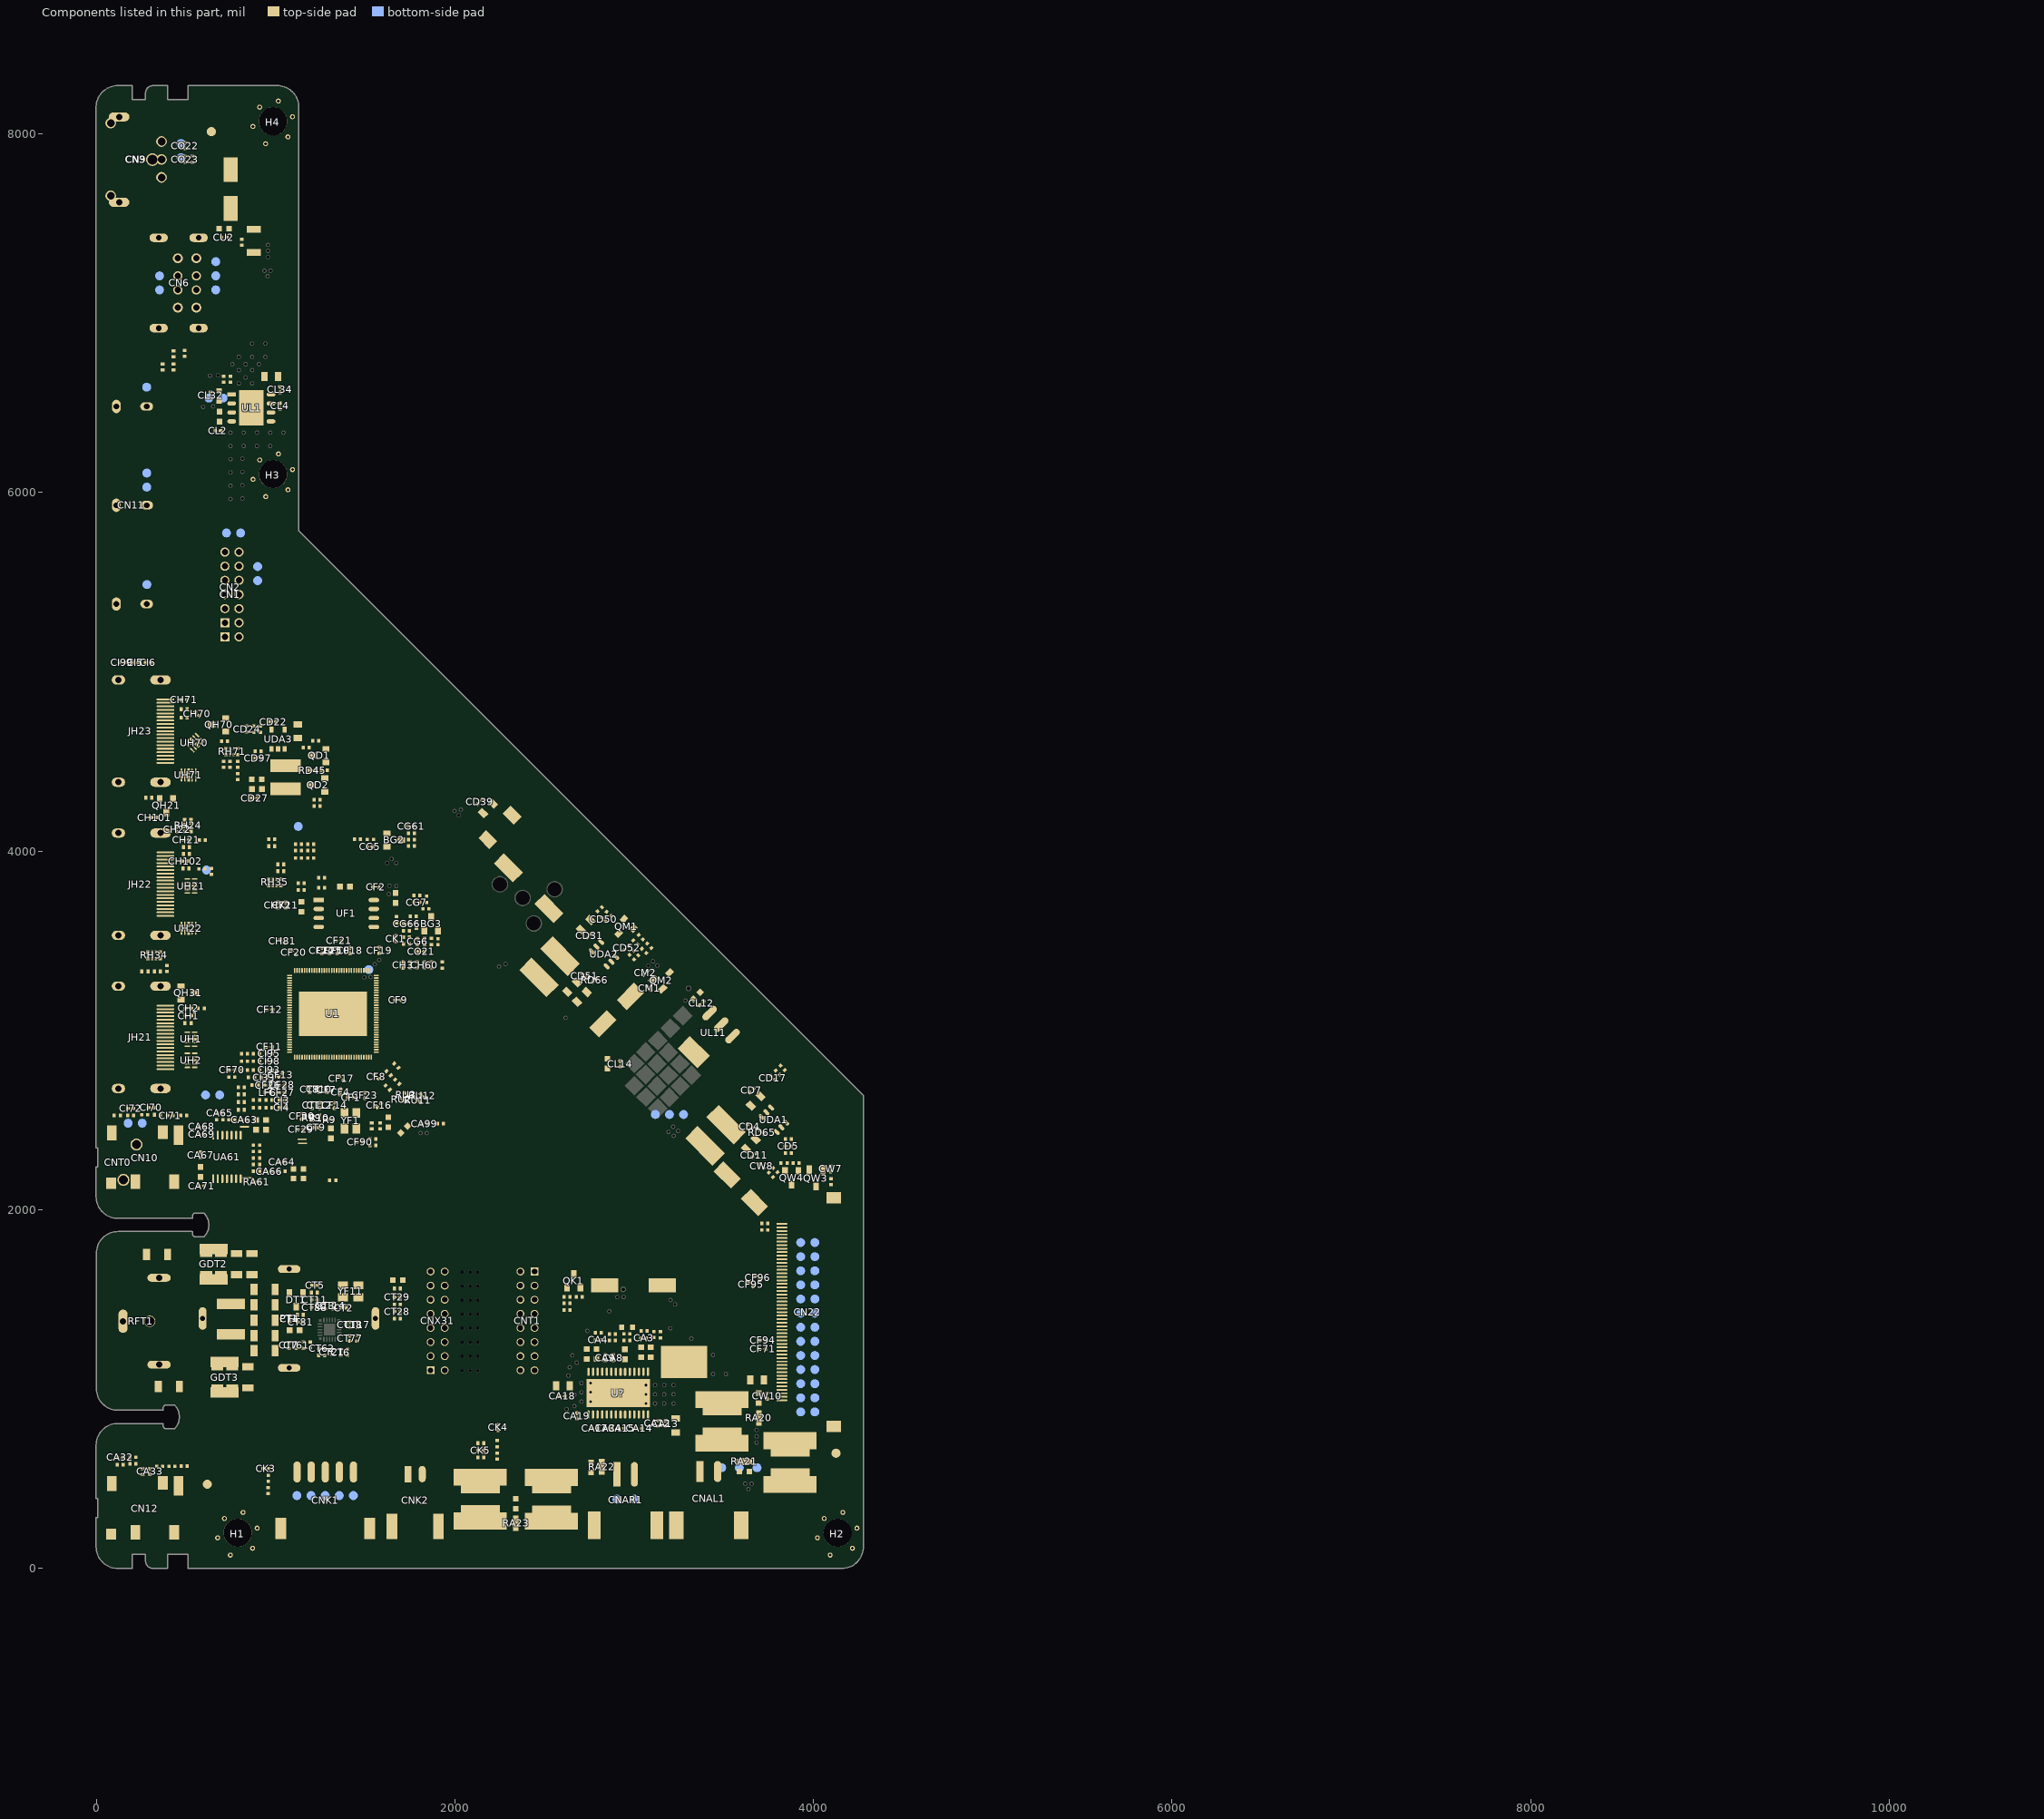
[diagram p0: the components of this part, seen from the top]
# Altium PCB MISC105950.PcbDoc (part 4 of 15)
Units mil, origin at the board's own origin, x right, y up, seen from the top; angles counter-clockwise.
Board outline 4280.62 x 8272.76 mil, 2 copper layers (TopLayer, BottomLayer), stack 61.855 mil thick; 541 components, 268 nets, 2324 pads, 1157 vias.

## Footprints (in the part's own frame and the unit in brackets; to place one, negate y for a bottom-side part, rotate by r counter-clockwise, add the part's x,y. Pads: shape width x height; smd on the part's side, far side on the other; paste and mask are expansions set on the pad) (continued)
QFN128/0.35-1 [mm] "Mstar,TSUMV53RWUT-Z1,18.11.16(19.03.30   减少外延焊盘长度）(19.04.23 更新钢网尺寸）（因温升修改为12宫格）"
  oct 2.2x1.9 on Top Paste: 0(-3.7,0) 0(-3.697,-2.145) 0(-3.697,2.145) 0(-1.253,-2.145) 0(-1.253,2.145) 0(-1.25,0) 0(1.247,-2.145) 0(1.247,2.145) 0(1.25,0) 0(3.697,-2.145) 0(3.697,2.145) 0(3.7,0)
  oct 2.2x1.9 on Top Solder: 0(-3.7,0) 0(-3.697,-2.145) 0(-3.697,2.145) 0(-1.253,-2.145) 0(-1.253,2.145) 0(-1.25,0) 0(1.247,-2.145) 0(1.247,2.145) 0(1.25,0) 0(3.697,-2.145) 0(3.697,2.145) 0(3.7,0)
  rect 0.7x0.22 smd paste-0.02 mask-0.035: 1(-6.151,5.425)
  oval 0.7x0.22 smd paste-0.02 mask-0.035: 2(-6.151,5.075) 3(-6.151,4.725) 4(-6.151,4.375) 5(-6.151,4.025) 6(-6.151,3.675) 7(-6.151,3.325) 8(-6.151,2.975) 9(-6.151,2.625) 10(-6.151,2.275) 11(-6.151,1.925) 12(-6.151,1.575) 13(-6.151,1.225) 14(-6.151,0.875) 15(-6.151,0.525) 16(-6.151,0.175) 17(-6.151,-0.175) 18(-6.151,-0.525) 19(-6.151,-0.875) 20(-6.151,-1.225) 21(-6.151,-1.575) 22(-6.151,-1.925) 23(-6.151,-2.275) 24(-6.151,-2.625) 25(-6.151,-2.975) 26(-6.151,-3.325) 27(-6.151,-3.675) 28(-6.151,-4.025) 29(-6.151,-4.375) 30(-6.151,-4.725) 31(-6.151,-5.075) 32(-6.151,-5.425) 65(6.151,-5.425) 66(6.151,-5.075) 67(6.151,-4.725) 68(6.151,-4.375) 69(6.151,-4.025) 70(6.151,-3.675) 71(6.151,-3.325) 72(6.151,-2.975) 73(6.151,-2.625) 74(6.151,-2.275) 75(6.151,-1.925) 76(6.151,-1.575) 77(6.151,-1.225) 78(6.151,-0.875) 79(6.151,-0.525) 80(6.151,-0.175) 81(6.151,0.175) 82(6.151,0.525) 83(6.151,0.875) 84(6.151,1.225) 85(6.151,1.575) 86(6.151,1.925) 87(6.151,2.275) 88(6.151,2.625) 89(6.151,2.975) 90(6.151,3.325) 91(6.151,3.675) 92(6.151,4.025) 93(6.151,4.375) 94(6.151,4.725) 95(6.151,5.075) 96(6.151,5.425)
  oval 0.22x0.7 smd paste-0.02 mask-0.035: 33(-5.425,-6.151) 34(-5.075,-6.151) 35(-4.725,-6.151) 36(-4.375,-6.151) 37(-4.025,-6.151) 38(-3.675,-6.151) 39(-3.325,-6.151) 40(-2.975,-6.151) 41(-2.625,-6.151) 42(-2.275,-6.151) 43(-1.925,-6.151) 44(-1.575,-6.151) 45(-1.225,-6.151) 46(-0.875,-6.151) 47(-0.525,-6.151) 48(-0.175,-6.151) 49(0.175,-6.151) 50(0.525,-6.151) 51(0.875,-6.151) 52(1.225,-6.151) 53(1.575,-6.151) 54(1.925,-6.151) 55(2.275,-6.151) 56(2.625,-6.151) 57(2.975,-6.151) 58(3.325,-6.151) 59(3.675,-6.151) 60(4.025,-6.151) 61(4.375,-6.151) 62(4.725,-6.151) 63(5.075,-6.151) 64(5.425,-6.151) 97(5.425,6.151) 98(5.075,6.151) 99(4.725,6.151) 100(4.375,6.151) 101(4.025,6.151) 102(3.675,6.151) 103(3.325,6.151) 104(2.975,6.151) 105(2.625,6.151) 106(2.275,6.151) 107(1.925,6.151) 108(1.575,6.151) 109(1.225,6.151) 110(0.875,6.151) 111(0.525,6.151) 112(0.175,6.151) 113(-0.175,6.151) 114(-0.525,6.151) 115(-0.875,6.151) 116(-1.225,6.151) 117(-1.575,6.151) 118(-1.925,6.151) 119(-2.275,6.151) 120(-2.625,6.151) 121(-2.975,6.151) 122(-3.325,6.151) 123(-3.675,6.151) 124(-4.025,6.151) 125(-4.375,6.151) 126(-4.725,6.151) 127(-5.075,6.151) 128(-5.425,6.151)
  rect 9.6x6.3 smd paste-6 mask-6: EPAD(0,0)
  silkscreen extent -7.48,-7.42 7.42,7.4, body extent -6.2,-6.2 6.2,6.2, height 0.95
R0402 [mm] "片式电阻"
  rect 0.45x0.5 smd mask+0.076: 1(-0.425,0) 2(0.425,0)
  silkscreen extent -0.8,-0.4 0.8,0.4, body extent -0.5,-0.25 0.5,0.25, height 0.5
R0402SC#1 [mm]
  rect 0.45x0.5 smd mask+0.076: 1(-0.425,0) 2(0.425,0)
  rect 0.42x0.25 smd paste-0.5 mask-0.5: 3(0,0)
  silkscreen extent -0.8,-0.4 0.8,0.4, body extent -0.5,-0.25 0.5,0.25, height 0.5
R0402SC#2 [mm]
  rect 0.45x0.5 smd mask+0.076: 1(-0.425,0) 2(0.425,0)
  rect 0.42x0.305 smd paste-0.5 mask-0.5: 3(0,0)
  silkscreen extent -0.8,-0.4 0.8,0.4, body extent -0.5,-0.25 0.5,0.25, height 0.5
R0603 [mm] "贴片电阻"
  rect 0.7x0.8 smd mask+0.076: 1(-0.756,0) 2(0.756,0)
  silkscreen extent -1.25,-0.54 1.25,0.54, body extent -0.8,-0.4 0.8,0.4, height 0.8
R0603SC [mm] "贴片电阻"
  rect 0.7x0.8 smd mask+0.076: 1(-0.756,0) 2(0.756,0)
  rect 0.82x1 smd paste-0.5 mask-0.5: 3(0,0)
  silkscreen extent -1.25,-0.54 1.25,0.54, body extent -0.8,-0.4 0.8,0.4, height 0.8
RA0402 [mm] "排阻"
  rect 0.5x0.5 smd mask+0.076: 1(-0.45,0.85) 2(0.45,0.85) 7(-0.45,-0.85) 8(0.45,-0.85)
  rect 0.5x0.3 smd mask+0.076: 3(-0.45,0.25) 4(0.45,0.25) 5(-0.45,-0.25) 6(0.45,-0.25)
  silkscreen extent -0.85,-1.27 0.85,1.27, body extent -0.51,-1 0.51,1, height 0.35
RCL0524P [mm] "RCLAMP0524J(19.03.04 优化丝印）"
  rect 0.21x0.8 smd: 1(-1,-0.52)
  oval 0.21x0.8 smd: 2(-0.5,-0.52) 3(0.5,-0.52) 4(1,-0.52) 5(1,0.52) 6(0.5,0.52) 7(-0.5,0.52) 8(-1,0.52)
  rect 0.38x0.8 smd: GND(0,0.52) GND(0,-0.52)
  silkscreen extent -1.4,-2.03 1.4,1.14, body extent -1.25,-0.6 1.25,0.6, height 0.66
SHIELD(24.5*14*6)-TEMP-NG [mm] "屏蔽罩"
  rect 2.8x5.5 on Top Paste mask+0.051: 0(-7,0) 0(7,0)
  rect 5.5x2.8 on Top Paste mask+0.051: 0(0,12.25) 0(0,-12.25)
  oval 3.2x1.1 hole 0.7 slot 2.8 at 0 deg mask+0.051: 1(0,12.25) 2(0,-12.25)
  oval 1.1x3.2 hole 0.7 slot 2.8 at 90 deg mask+0.051: 3(7,0) 4(-7,0)
  silkscreen extent -7.48,-13.1 7.51,13.1, body extent -7.53,-13.17 7.53,13.16, height 6.1
SIP2*6H/2.0D-LS [mm] "新富尔，PHD-2*6AW-DK-SMT-P，带扣、台阶。XXXXXXXXXXXXXX项目用，17.08.16"
  rect 1.75x2.45 on Top Paste: 0(-5,-1.365) 0(-5,1.388) 0(-3,-1.364) 0(-3,1.388) 0(-1,-1.364) 0(-1,1.388) 0(1,-1.365) 0(1,1.388) 0(3,1.388) 0(3,-1.365) 0(5,-1.365) 0(5,1.388)
  rect 1.3x1.3 hole 0.9 mask+0.076: 1(-5,0.788)
  round 1.3 hole 0.9 mask+0.076: 2(-5,-1.212) 3(-3,0.788) 4(-3,-1.212) 5(-1,0.788) 6(-1,-1.212) 7(1,0.787) 8(1,-1.212) 9(3,0.788) 10(3,-1.212) 11(5,0.788) 12(5,-1.212)
  silkscreen extent -7.82,-9.54 7.1,2.41
SIP2*7H/2.0D-LS [mm] "新富尔，PHD-2*7AW-DK-SMT-P，带卡扣、台阶。XXXXXXXXXXXXXX项目用，17.08.16"
  rect 1.75x2.45 on Top Paste: 0(-6,-1.365) 0(-6,1.388) 0(-4,-1.364) 0(-4,1.388) 0(-2,-1.364) 0(-2,1.388) 0(0,1.388) 0(0,-1.365) 0(2,1.388) 0(2,-1.365) 0(4,-1.365) 0(4,1.388) 0(6,-1.364) 0(6,1.388)
  rect 1.3x1.3 hole 0.9 mask+0.076: 1(-6,0.788)
  round 1.3 hole 0.9 mask+0.076: 2(-6,-1.212) 3(-4,0.788) 4(-4,-1.212) 5(-2,0.788) 6(-2,-1.212) 7(0,0.787) 8(0,-1.212) 9(2,0.788) 10(2,-1.212) 11(4,0.788) 12(4,-1.212) 13(6,0.788) 14(6,-1.212)
  silkscreen extent -8.82,-9.54 8.1,2.41
SIP2*8H/2.0DF-1 [mm] "东莞龙科；130-F1628210-B91;15.02.06"
  round 1.3 on Top Overlay: 0(-7,-1) 0(-5,-1) 0(-5,1) 0(-3,-1) 0(-3,1) 0(-1,-1) 0(-1,1) 0(1,-1) 0(1,1) 0(3,-1) 0(3,1) 0(5,-1) 0(5,1) 0(7,-1) 0(7,1)
  rect 1.3x1.3 on Top Overlay: 0(-7,1)
  rect 1.1x1.1 hole 0.8: 1(-7,1)
  round 1.1 hole 0.8: 2(-7,-1) 3(-5,1) 4(-5,-1) 5(-3,1) 6(-3,-1) 7(-1,1) 8(-1,-1) 9(1,1) 10(1,-1) 11(3,1) 12(3,-1) 13(5,1) 14(5,-1) 15(7,1) 16(7,-1)
  silkscreen extent -8.75,-8.9 8.35,2.54, body extent -8.25,-8.8 8.25,1.2, height 6.03
SIP2*8H/2.0DM-1 [mm] "东莞龙科；142-M1628210-B31;15.02.06"
  round 1.3 on Top Overlay: 0(-7,-1) 0(-5,-1) 0(-5,1) 0(-3,1) 0(-3,-1) 0(-1,1) 0(-1,-1) 0(1,1) 0(1,-1) 0(3,1) 0(3,-1) 0(5,-1) 0(5,1) 0(7,-1) 0(7,1)
  rect 1.3x1.3 on Top Overlay: 0(-7,1)
  rect 1.1x1.1 hole 0.8: 1(-7,1)
  round 1.1 hole 0.8: 2(-7,-1) 3(-5,1) 4(-5,-1) 5(-3,1) 6(-3,-1) 7(-1,1) 8(-1,-1) 9(1,1) 10(1,-1) 11(3,1) 12(3,-1) 13(5,1) 14(5,-1) 15(7,1) 16(7,-1)
  silkscreen extent -11.73,-7.87 11.73,2.54, body extent -11.6,-7.77 11.6,1.23, height 5.5
SIP2H/2.0S-3 [mm] "捷仕泰/铭锋达/创佳；2PIN-2.0-L-M-G-带扣-带台阶-C；14.07.28"
  rect 1x2.3 smd: 1(-1,3.7)
  oval 1x2.3 smd: 2(1,3.7)
  rect 1.5x3.6 smd: 3(-3.3,-3.7) 4(3.3,-3.7)
  silkscreen extent -4.13,-5.15 4.13,4.15
SIP2H/2.5S-3 [mm] "新富尔；XH-2AWB-DK-R;插线高度为9.8mm;15.08.31"
  rect 1x3.5 smd: 1(-1.25,1)
  oval 1x3.5 smd: 2(1.25,1)
  rect 1.8x3.9 smd: 3(4.45,-6.2) 4(-4.45,-6.2)
  silkscreen extent -5.13,-7.95 5.13,0.05
SIP2H/2.5S-4 [mm] "正理；TJC3B-2AW(插线后高度8.5mm)；160607"
  rect 1x3 smd: 1(-1.25,1.4)
  oval 1x3 smd: 2(1.25,1.4)
  rect 2.1x3.9 smd: 3(4.6,-6.2) 4(-4.6,-6.2)
  silkscreen extent -5.15,-7.95 5.15,0.1
SIP5H/2.0S-4 [mm] "浙江正理；2008-nAW-S;15.07.27(17.06.16缩小优化地脚焊盘）"
  oval 1x3 smd: 1(-4,4) 2(-2,4) 3(0,4) 4(2,4) 5(3.997,3.997)
  rect 1.5x3 smd: 6(6.3,-4) 7(-6.3,-4)
  silkscreen extent -7.18,-5.27 7.18,4.1, body extent -7,-5.1 7,5, height 5.18
SMD4532-1 [mm] "Brightking,4532-091-LF,气体放电管,雷电防护器件，17.06.12"
  rect 1.5x4 smd: 1(-2.15,0) 2(2.151,0)
  silkscreen extent -1.25,-1.79 1.23,1.71, body extent -2.41,-1.75 2.41,1.75, height 3
SMD4532-1-C1206 [mm] "Brightking,4532-091-LF,SMD4532-1兼容C1206封装，19.01.08"
  rect 1.6x1 smd paste-5 mask-5: 1(-1.016,-1.501) 1(1.016,-1.499) 2(-1.016,1.501) 2(1.016,1.501)
  rect 1.6x1 on Top Paste paste-5 mask-5: 1(-1.016,-1.501) 1(1.016,-1.501) 2(-1.016,1.501) 2(1.016,1.501)
  rect 4x1.5 smd paste-5 mask-5: 1(0,-2.15) 2(0,2.151)
  rect 4.001x0.903 on Top Paste: 1(0.05,-2.499) 2(0.05,2.499)
  silkscreen extent -1.96,-1.16 1.96,1.2, body extent -1.82,-2.41 1.81,2.41, height 3
SO-23 [mm] "双向二极管封装"
  rect 0.8x1 smd: 1(0.952,1.016) 3(-0.953,1.016)
  rect 0.8x1.1 smd: 2(0,-0.966)
  silkscreen extent -1.55,-0.86 1.55,0.36, body extent -1.5,-1.25 1.5,1.25, height 1.1
SOIC8 [mm] "W25X40BVSNIG/GD25Q32BSIG/GD25LQ16"
  rect 1.5x0.6 smd: 1(-3.9,1.905)
  oval 1.5x0.6 smd: 2(-3.9,0.635) 3(-3.9,-0.635) 4(-3.9,-1.905) 5(3.9,-1.905) 6(3.9,-0.635) 7(3.9,0.635) 8(3.9,1.905)
  silkscreen extent -5.71,-2.65 2.7,2.65, body extent -4.05,-2.69 4.05,2.69, height 2.17
SOP8/1.27-3 [mm] "LEADCHIP;LC1118;14-05-09"
  rect 1.238x0.6 smd: 1(-2.782,1.905)
  oval 1.238x0.6 smd: 2(-2.782,0.635) 3(-2.782,-0.635) 4(-2.782,-1.905) 5(2.783,-1.905) 6(2.783,-0.635) 7(2.782,0.635) 8(2.782,1.905)
  rect 3.5x5 smd paste-3 mask-3: EPAD(0,0)
  silkscreen extent -3.1,-2.5 4.16,3.16, body extent -3.1,-2.5 3.1,2.5, height 1.76
SOT23-6-2 [mm] "ONSEMI;  NL27WZU04"
  oval 0.5x1 smd: 1(-0.95,-1.5) 2(0,-1.5) 3(0.95,-1.5) 4(0.95,1.5) 5(0,1.5) 6(-0.95,1.5)
  silkscreen extent -2.21,-2.18 1.55,0.85, body extent -1.55,-0.85 1.55,0.85, height 1.2
SOT-23 [mm]
  rect 0.8x1 smd: B(0.953,1.016) E(-0.952,1.016)
  rect 0.8x1.1 smd: C(-0.013,-0.966)
  silkscreen extent -1.55,-0.81 1.55,0.36, body extent -1.5,-1.25 1.5,1.25, height 1.1
SOT-23-1 [mm]
  rect 0.8x1.1 smd: D(0,-1.15)
  rect 0.8x1.27 smd: G(0.95,1.2) S(-0.95,1.2)
  TopLayer pour cut-out: -1.583,0.903 -1.583,-0.905 1.587,-0.905 1.587,0.903
  silkscreen extent -1.55,-1.05 1.55,0.33, body extent -1.52,-1.48 1.52,1.48, height 1.25
SOT-23-5 [mm] "LPW5206(1.295mm)"
  rect 0.6x0.8 smd: 1(-0.95,-1.375) 2(0,-1.375) 3(0.95,-1.375) 4(0.95,1.375) 5(-0.95,1.375)
  silkscreen extent -2.29,-1.16 1.5,0.85, body extent -1.5,-0.85 1.5,0.85, height 1.45
SOT-223 [mm]
  oval 1x2.5 smd: 1(-2.3,-2.75) 2(0,-2.75) 3(2.3,-2.75)
  rect 4x2.5 smd: 4(0,2.75)
  TopLayer pour cut-out: 2.3,-1.188 2.3,-4.312 -2.345,-4.312 -2.64,-4.253 -2.891,-4.086 -3.058,-3.835 -3.117,-3.54 -3.117,-3.54 -2.299,-3.54 -2.299,-1.956 -3.124,-1.956 -3.066,-1.662 -2.899,-1.413 -2.65,-1.247 -2.356,-1.188 -2.356,-1.188
  silkscreen extent -3.45,-2.75 3.45,2.81, body extent -3.35,-3.3 3.35,3.4, height 1.7
SSOP14/0.65-1 [mm] "TI,MSP430G2001"
  oval 0.3x1.225 smd: 1(-1.95,-3.087) 2(-1.3,-3.087) 3(-0.65,-3.087) 4(0,-3.087) 5(0.65,-3.087) 6(1.3,-3.087) 7(1.95,-3.087) 8(1.95,3.088) 9(1.3,3.088) 10(0.65,3.088) 11(0,3.088) 12(-0.65,3.088) 13(-1.3,3.088) 14(-1.95,3.088)
  silkscreen extent -2.55,-4.7 2.55,4.6, body extent -2.55,-3.19 2.55,3.19, height 1.2
SSOP28/0.65-5 [mm] "TI;TPA3140D2PWPR;15.07.08"
  rect 1.15x0.34 smd mask+0.076: 1(-3.025,4.225)
  oval 1.15x0.34 smd mask+0.076: 2(-3.025,3.575) 3(-3.025,2.925) 4(-3.025,2.275) 5(-3.025,1.625) 6(-3.025,0.975) 7(-3.025,0.325) 8(-3.025,-0.325) 9(-3.025,-0.975) 10(-3.025,-1.625) 11(-3.025,-2.275) 12(-3.025,-2.925) 13(-3.025,-3.575) 14(-3.025,-4.225) 15(3.025,-4.225) 16(3.025,-3.575) 17(3.025,-2.925) 18(3.025,-2.275) 19(3.025,-1.625) 20(3.025,-0.975) 21(3.025,-0.325) 22(3.025,0.325) 23(3.025,0.975) 24(3.025,1.625) 25(3.025,2.275) 26(3.025,2.925) 27(3.025,3.575) 28(3.025,4.225)
  oct 1.05x1.318 on Top Paste mask+0.076: EPAD(-0.675,2.427) EPAD(-0.675,0.809) EPAD(-0.675,-0.809) EPAD(-0.675,-2.427) EPAD(0.675,2.427) EPAD(0.675,0.809) EPAD(0.675,-0.809) EPAD(0.675,-2.427)
  oct 1.05x1.318 on Top Solder mask+0.076: EPAD(-0.675,2.427) EPAD(-0.675,0.809) EPAD(-0.675,-0.809) EPAD(-0.675,-2.427) EPAD(0.675,2.427) EPAD(0.675,0.809) EPAD(0.675,-0.809) EPAD(0.675,-2.427)
  rect 4x9 smd paste-5 mask-5: EPAD(0,0)
  silkscreen extent -4.65,-4.9 4.64,4.9, body extent -2.25,-4.9 2.25,4.9, height 1.2
T-12.8×10×9.3-IEC14.5-6.3 [mm] "GD.120-XX1.09/26/2019"
  rect 3.3x4.6 on Top Paste: 0(-6.15,8.851) 0(6.15,8.851)
  rect 3.3x3.3 on Top Paste: 0(0,7.731)
  rect 4.6x3.3 on Top Paste: 0(0,3.751)
  round 1.6 hole 1.4: 1(0,7.531)
  oval 3.3x1.3 hole 0.9 slot 2.7 at 0 deg: 2(0,3.751)
  oval 1.1x3.3 hole 0.9 slot 2.7 at 90 deg: 3(-6.15,8.851) 4(6.15,8.851)
  silkscreen extent -7.55,-0.05 7.55,13.62
TP [mil] "TEST POINT   (不带paste  1.27mm 直径）"
  round 50 smd: 1(0,0)
USB2-HS-1 [mm] "WCLO,WLUS-364A,通孔回流，17.11.17"
  rect 3.2x4.4 on Top Paste: 0(-7.255,13.46) 0(-7.255,8.3) 0(7.255,13.46) 0(7.255,8.3)
  rect 1.8x3.5 on Top Paste: 0(-3.5,14.192) 0(-3.5,10.448) 0(-1.025,14.192) 0(-1.025,10.448) 0(1.025,14.192) 0(1.025,10.448) 0(3.5,14.192) 0(3.5,10.448)
  round 1.4 hole 0.9 mask+0.076: 1(-3.5,13.63) 4(3.5,13.63) 5(-3.5,11.01) 8(3.5,11.01)
  round 1.3 hole 0.9 mask+0.076: 2(-1,13.63) 3(1,13.63) 6(-1,11.01) 7(1,11.01)
  oval 1.2x2.6 hole 0.8 slot 2.2 at 90 deg mask+0.076: 9(-6.4,13.96) 10(6.4,13.96) 11(-6.4,8.3) 12(6.4,8.3)
  KeepOutLayer pour cut-out: -5.206,11.033 -5.206,13.649 -4.578,13.021 -4.578,11.669 -5.214,11.033
  KeepOutLayer pour cut-out: -3.49,12.749 -3.574,12.749 -3.826,12.724 -4.149,12.626 -4.447,12.467 -4.709,12.252 -4.923,11.991 -5.083,11.693 -5.181,11.369 -5.206,11.117 -5.206,11.033 -5.206,11.033 -5.206,10.993 -5.206,10.905 -5.179,10.64 -5.076,10.3 -4.909,9.987 -4.684,9.712 -4.409,9.487 -4.096,9.319 -3.756,9.216 -3.491,9.19 -3.402,9.19 -3.402,9.19 2.42,9.19 2.476,9.19 2.641,9.223 2.829,9.348 2.954,9.535 2.986,9.7 2.986,9.756 2.986,9.756 2.986,12.202 2.986,12.256 2.954,12.418 2.832,12.602 2.648,12.724 2.487,12.756 2.432,12.756 2.432,12.756 -3.482,12.756 -3.484,12.756 -3.488,12.755 -3.49,12.75 -3.49,12.749
  KeepOutLayer pour cut-out: -3.49,15.369 -3.574,15.369 -3.826,15.344 -4.149,15.246 -4.447,15.087 -4.709,14.872 -4.923,14.611 -5.083,14.313 -5.181,13.989 -5.206,13.737 -5.206,13.653 -5.206,13.653 -5.206,13.613 -5.206,13.525 -5.179,13.26 -5.076,12.92 -4.909,12.607 -4.684,12.332 -4.409,12.107 -4.096,11.939 -3.756,11.836 -3.491,11.81 -3.402,11.81 -3.402,11.81 2.42,11.81 2.476,11.81 2.641,11.843 2.829,11.968 2.954,12.155 2.986,12.32 2.986,12.376 2.986,12.376 2.986,14.822 2.986,14.876 2.954,15.038 2.832,15.222 2.648,15.344 2.487,15.376 2.432,15.376 2.432,15.376 -3.482,15.376 -3.484,15.376 -3.488,15.375 -3.49,15.37 -3.49,15.369
  silkscreen extent -6.7,0 6.7,15.25, body extent -7.5,-1.98 7.5,15.17, height 16.05
XTAL-S-3 [mm] "三星（SQ3D03200D2IBA）晶振"
  rect 1.4x1.1 smd: 1(-1.1,-0.85) 2(1.1,-0.85) 3(1.1,0.85) 4(-1.1,0.85)
  silkscreen extent -2.37,-1.91 1.65,1.3, body extent -1.65,-1.3 1.65,1.3, height 0.8

## Part data
5V 5V_IR DM0 DM1 DP0 DP1 GND_AMP GND_KEY IR KEY LED LOUT+ LOUT- ROUT+ ROUT- RXD TXD: library part TEST
BG2 BG3 QD2: library part LMBT3904LT1G-D-NPN, "Q-NPN-#-#-#"
CA1 CA2 CD53 CD54 CD57 CL10 CW9: library part 004.003.0000386-D, "Ceramic capacitor, CAP MC, 16V, 10uF, ±20%, X5R, 0805, SMD, TP-D"
CA3 CA4: library part 004.003.0000549-D, "Ceramic capacitor, CAP MC, 50V, 3300pF, ±10%, X7R, 0402, SMD, TP-D"
CA5 CA6 CA10 CA11: library part 004.003.0000400-D, "Ceramic capacitor, CAP MC, 16V, 0.22uF, ±10%, X5R, 0603, SMD, TP-D"
CA7 CA20 CA21 CA22 CA23: library part 1uF-0603-X7R-±10%-10V-D
CA8 CA12 CA18 CA69 CD4 CD51 CI3 CI4 CK4 CK5 CL2 CL12 CL32 CM1 CM2 CO22 CT1 CT9 CT12: library part 004.003.0000403-D, "Ceramic capacitor, CAP MC, 16V, 0.1uF, ±20%, X5R, 0402, SMD, TP-D"
CA9: library part 004.003.0000402-D, "Ceramic capacitor, CAP MC, 16V, 1uF, ±20%, X5R, 0402, SMD, TP-D"
CA13 CA19: library part 004.003.0000503-D, "Ceramic capacitor, CAP MC, 50V, 1000pF, ±10%, X7R, 0402, SMD, TP-D"
CA14 CA15 CA17 CA34: library part 004.003.0000398-D, "Ceramic capacitor, CAP MC, 16V, 0.22uF, ±20%, X5R, 0402, SMD, TP-D"
CA29 CA31 CA59 CA60: library part 22uF-0603-X5R-±20%-6.3V-D
CA32 CA33 CA63 CA64 CA67 CL14: library part 004.003.0000382-D, "Ceramic capacitor, CAP MC, 6.3V, 1uF, ±20%, X5R, 0402, SMD, TP-D"
CA65 CA66: library part 004.003.0000532-D, "Ceramic capacitor, CAP MC, 50V, 220pF, ±5%, NPO, 0402, SMD, TP-D"
CA68: library part 004.003.0000100-D, "Ceramic capacitor, CAP MC, 6.3V, 2.2uF, ±20%, X5R, 0402, SMD, TP-D"
CA70 CF3 CF5 CF6 CF15 CF58 CF59 CL13 CT80 CU1: library part 004.003.0000383-D, "Ceramic capacitor, CAP MC, 6.3V, 10uF, ±20%, X5R, 0603, SMD, TP-D"
CA71 CD22 CD27 CG5 CG6 CG7 CG61 CH1 CH2 CH3 CH21 CH22 CH60 CH70 CH71 CH72 CW7 CW10: library part 0.1uF-0402-X5R-±20%-16V-D
CA99 CF11 CF16 CF18 CF19 CF20 CF21 CF23 CF24 CF25 CF28 CG66 CH81 CL4 CL34 CT5 CU2: library part 1uF-0402-X5R-±20%-6.3V-D
CD5 CD52: library part 004.003.0000558-D, "Ceramic capacitor, CAP MC, 50V, 470pF, ±5%, NPO, 0402, SMD, TP-D"
CD7 CD17 CD31 CD39 CD50: library part 004.003.0000814-D, "Ceramic capacitor, CAP MC, 25V, 0.1uF, ±20%, X5R, 0402, SMD, TP-D"
CD11 CD97 CF2 CF7 CF8 CF9 CF10 CF12 CF13 CF14 CF17 CF27 CK3 CT2 CT3 CT4 CT7 CT11 CT14 CT17 CT18 CT21 CT61 CT62 CT81 CT88: library part 0.1uF-0402-Y5V-+80%-20%-16V-D
CD24: library part 3300pF-0402-X7R-±10%-50V-D
CD25 CD26: library part 10uF-0603-X5R-±20%-6.3V-D
CD30 CD77 CD96: library part 10uF-0805-X5R-+15%-16V-D
CD99: library part 10uF-0805-X5R-±20%-16V-D
CD101 CD102 DH73 DH74 DH75 DH76 DK2 DK3 DK4: library part AVLC18S02003-D
CF1 CF4: library part 30pF-0402-NPO-±5%-50V-D
CF26 CF70: library part 0.047uF-0402-X7R-±10%-16V-D
CF29 CF30 CF90: library part 1000pF-0402-X7R-±10%-50V-D
CF71 CF94 CF95 CF96: library part 5pF-0402-NPO-±5%-50V-D
CH101 CH102: library part 220pF-0402-X7R-±10%-50V-D
CI5 CI6 CI70 CI71 CI72 CI99: library part 004.003.0000500-D, "Ceramic capacitor, CAP MC, 50V, 10pF, ±5%, NPO, 0402, SMD, TP-D"
CI33 CI93 CI95 CI98: library part 004.003.0000562-D, "Ceramic capacitor, CAP MC, 16V, 0.047uF, ±10%, X7R, 0402, SMD, TP-D"
CK1: library part 22pF-0402-NPO-±5%-50V-D
CK11: library part 0.01uF-0402-X7R-±10%-50V-D
CL1 CL11 CL31: library part 004.003.0000394-D, "Ceramic capacitor, CAP MC, 10V, 10uF, ±20%, X5R, 0603, SMD, TP-D"
CN1: library part XXX.XXX.0003725, "Connector socket, connect jack, 2×7PIN, D2.0, L, SNAP, STEP, Fool-proofing, Nature, L=2.5, SMD, PHD-2*7AW-DK-SMT-P, XFE-D"
CN2: library part XXX.XXX.0003724, "Connector socket, connect jack, 2×6PIN, D2.0, L, SNAP, STEP, Fool-proofing, Nature, L=2.5, SMD, PHD-2*6AW-DK-SMT-P, XFE-D"
CN3: library part XXX.XXX.0004399-D, "RCA jack, RCA Jack, AV1, H, Orange, CH5.5, Seal, SMD, RCA-143P1-EP-07, CS-D"
CN6: library part PKG-003697/P000082044, "USB jack, USB2.0, H, Double, flange, SMD, WLUS-364A, WCLO-D"
CN9: library part XXX.XXX.0002412, "Optical jack, OPTICAL, H, SMD, 182500122, VAST-D"
CN10 CN12: library part XXX.XXX.0004228-D, "Earphone jack, Earphone Jack, H, Φ3.5, CH2.25, Black, switch, Seal, SMD, PJ-342F, JSL-D"
CN11: library part XXX.XXX.0003918-D, "RCA jack,RCA Jack,AV3,H,Yellow,White,Red,CH5.5,D14,Seal,SMD-L,AⅤ-8.4-16A yellow/white/red,JSL-D"
CN22: library part "FFC插座,FFC connector,51Pin,D0.5,Bottom,lock,SMD,CT-D", "CN-FFC socket, flip-cover"
CNAL1: library part XXX.XXX.0001786-D, "Connector socket, connect jack, 2pin, D2.5, L, SNAP, Fool-proofing, Nature, L=2.4mm, SMD, AMA-D"
CNAR1: library part 连接插座,2PIN,D2.5,L,SNAP,Fool-proofing,RED,SMD,XFE-D
CNK1: library part XXX.XXX.0001782, "Connector socket, connect jack, 5pin, D2.0, L, SNAP, STEP, Fool-proofing, Nature, L=2.5mm, SMD, AMA-D"
CNK2: library part XXX.XXX.0002231, "Connector socket, connect jack, 2Pin, D2.0, L, SNAP, STEP, Fool-proofing, Nature, SMD, 2008-2AW-S, AMA-D"
CNT0: library part PKG-004688/P000102833-D, "Standoff, Φ5.5×7.0×7.8mm-M3, nickel-plated, iron, SMT-D"
CNT1: library part "连接插座-公座,male connect jack,2×8Pin,D2.0,L,Fool-proofing,Black,L=3.0mm,DIP,LK-DLMI"
CNX31: library part "连接插座-母座,female connect jack,2×8Pin,D2.0,L,Fool-proofing,Black,L=2.6mm,DIP,LK-DLMI"
CO21: library part 004.003.0000546-D, "Ceramic capacitor, CAP MC, 50V, 33pF, ±5%, NPO, 0402, SMD, TP-D"
CO23: library part 004.003.0000045-D, "Ceramic capacitor, CAP MC, 50V, 330pF, ±5%, NPO, 0402, SMD, TP-D"
CT6 CT77: library part 004.003.0000530-D, "Ceramic capacitor, CAP MC, 50V, 22pF, ±5%, NPO, 0402, SMD, TP-D"
CT8 CT10 CT28 CT29: library part 004.003.0000556-D, "Ceramic capacitor, CAP MC, 50V, 47pF, ±5%, NPO, 0402, SMD, TP-D"
CT40: library part 0.47uF-1206-Y5V-+80%-20%-16V-D
CT41 CT42 CT43 CT44 CT45 CT46 CT47 CT48 CT49 CT50 CT51 CT52 CT53: library part 1000pF-1206-X7R-±20%-2000V-D
CW8: library part 0.022uF-0402-X7R-±10%-16V-D
DA51 DA52 DA53 DH1 DH2 DH3 DH4 DH21 DH22 DH23 DH70 DH71 DH72 DH81 DI2 DI3 DI22 DI23 DI24 DI33 DI34 DO21: library part 004.005.0000315-D, "TVS diode, DIO ESD, 2.5pF, 200V, 0402, SMD, SFI0402-240E-2R5PP-LF, SFI-D"
DAS1: library part DOLBY_AS2
DK70: library part SFI0402-240E-2R5PP-LF-D
DM4: library part 004.005.0000611, "TVS diode, DIO ESD, 19.9V, SMB, SMD, SMBFJ12A, LRC-D"
DT1: library part BAV99-BR-D
DU1 DU2 DU11 DU12 DU31 DU32 DU33 DU34: library part 004.005.0000203-D, "TVS diode, DIO ESD, 0.2pF, 25V, 0402, SMD, AIES12U020R2, AMOTECH-D"
EA1 ED6 EU1: library part 004.003.0000405-D, "Aluminum electrolytic capacitor, CAP AL, 16V, 100uF, ±20%, HV, P, 6.3×5.5, SMD, TP, CapXon-D"
EA33 EA34: library part "铝电解电容,CAP AL,100V,33uF,±20%,LF,RV,10×10.5,SMD,TP,CapXon-D", "Electrolytic"
FT2 LT2 LT3 LT4: library part SDCL1005CR27JTDF(顺络)-D
FU1: library part 004.026.0000039-D, "Resettable fuse, FUSE PTC, 1.1A, 6V, 1206, SMD, TP, TLC-D"
GDT1: library part 004.005.0000675, "Gas discharge tube, GDT, 700V, 2000A, TP, 4.5*3.2mm, SMD, 4532-091-LF, Brightking-D"
GDT2 GDT3: library part 004.005.0000675-C1206, "Gas discharge tube, GDT, 700V, 2000A, TP, 4.5*3.2mm, SMD, 4532-091-LF, Brightking-D"
H1 H2 H3 H4: library part "Location hole-D"
HS1: library part 004.040.0008928-D, "Heatsink, 15.0×15.0×5.0mm, AL1060H-24, black, high-emissivity paint spray, stamped with bends, no rivet legs, YT-D"
HSA1: library part 17.5×14.5×0.5-本色-Cu-MRD-D, "Heatsink"
JH21 JH22 JH23: library part 161031041(外壳SPCC)-D, "CN-HDMI-horizontal-#-#"
LA1 LA3 LA6 LA8: library part 004.004.0000054-D, "Power inductor, Power Inductor, 15uH, ±20%, 2.60A, DR8.0×4.0, SMD, SWPA8040S150MT, Sunlord-D"
LA2 LA4 LA5 LA7: library part SMD5845-220M-03-1-HLY-D
LD1 LD11: library part 004.004.0000017-D, "Power inductor, Power Inductor, 4.7uH, ±20%, 2.8A, 0.35×1P, DR5.8×4.5, SMD, SCD54TL-4R7M, Soldier-D"
LD21: library part SLN43T-6R8M-D
LF6 R9 R10 R99 RA61 RD45 RD65 RD66 RU2 RU3 RU11 RU12: library part 0ohm-0402-PCB-D, "0ohm-0402-PCB-D"
LT1: library part 004.004.0000335-D, "Ferrite bead,BEAD,120ohm,0402,500mA,SMD,TP,GZ1005U121CTF,Sunlord-D"
LT80: library part MGLB1608M121T2R0-LF(120ohm-2000mA)-D
M1 M2 M3: library part MARK-D
PT1: library part 004.040.0007718-DLMI, "MB shield cover 2, D716AF, 48.9×33.9×3.3mm, SPET, natural color, QX-DLMI"
QD1: library part LMBT3906LT1G-D-PNP
QH21 QH31 QH70 QK1 QM1 QW4: library part 004.006.0000007-D, "General-purpose transistor, Dynatron, NPN, 0.2A, 40V, 60-300, SOT-23, KMBT3904, KEXIN-D"
QM2: library part 004.007.0000286-D, "MOSFET, PMOS, -4.7A, -20V, 70mohm@ID=-4.7A@VGS=-4.5V, SOT23-LC, LPB3443LT1G, LRC-D"
QW3: library part 004.007.0000281-D, "MOSFET, PMOS, -4.3A, -30V, 0.078ohm@ID=-3A@VGS=-4.5V, SOT-23, AO3487, AOS-D"
RA1 RA2 RA69 RA71 RM3 RW10 RW11: library part 004.002.0000689-D, "Thick-film resistor, RES, 1/16W, 4.7Kohm, ±5%, 0402, SMD-D"
RA3 RA14 RA55 RA56 RA68 RK10: library part 004.002.0000572-D, "Thick-film resistor, RES, 1/16W, 1Kohm, ±5%, 0402, SMD-D"
RA4 RA5 RA64 RA65: library part GND
RA6 RA15: library part 004.002.0000715-D, "Thick-film resistor, RES, 1/16W, 5.1ohm, ±5%, 0402, SMD-D"
RA7: library part 004.002.0000200-D, "Thick-film resistor, RES, 1/10W, 10Kohm, ±1%, 0603, SMD-D"
RA8 RA66 RA67 RD1 RD28 RD52 RD53 RM4: library part 004.002.0000579-D, "Thick-film resistor, RES, 1/16W, 100Kohm, ±5%, 0402, SMD-D"
RA9 RA51 RA62 RA63: library part 004.002.0000691-D, "Thick-film resistor, RES, 1/16W, 47Kohm, ±5%, 0402, SMD-D"
RA10: library part 004.002.0000575-D, "Thick-film resistor, RES, 1/16W, 10Kohm, ±1%, 0402, SMD-D"
RA11: library part 004.002.0000602-D, "Thick-film resistor, RES, 1/16W, 15Kohm, ±1%, 0402, SMD-D"
RA20 RA21 RA22 RA23: library part 0ohm-0603-PCB-D, "0ohm-0603-PCB-D"
RA52 RK15 RM1 RM2: library part 004.002.0000577-D, "Thick-film resistor, RES, 1/16W, 10Kohm, ±5%, 0402, SMD-D"
RA70 RA72: library part 004.002.0000589-D, "Thick-film resistor, RES, 1/16W, 12Kohm, ±5%, 0402, SMD-D"
RD2 RD44 RD46 RD47 RI13 RI15 RW14: library part 10Kohm-0402-±5%-1/16W-D
RD31 RD91: library part 004.002.0000104-D, "Thick-film resistor, RES, 1/16W, 33Kohm, ±1%, 0402, SMD-D"
RD35 RD54: library part 004.002.0000717-D, "Thick-film resistor, RES, 1/16W, 6.04Kohm, ±1%, 0402, SMD-D"
RD42 RG1 RG2: library part 510ohm-0402-±5%-1/16W-D